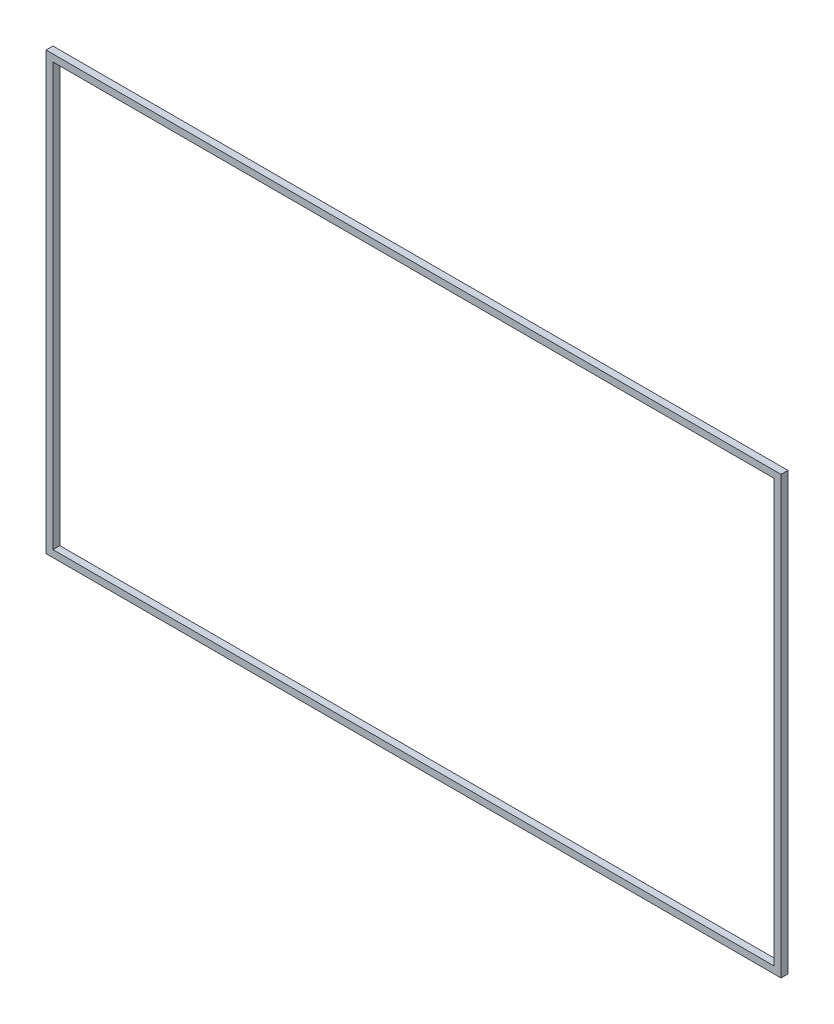
SolidWorks part; units mm, degrees
ref_plane "前视基准面" through (0, 0, 0) normal (0, 0, 1) x (1, 0, 0)
ref_plane "上视基准面" through (0, 0, 0) normal (0, 1, 0) x (1, 0, 0)
ref_plane "右视基准面" through (0, 0, 0) normal (1, 0, 0) x (0, 0, -1)
sketch "草图1" plane through (0, 0, 0) normal (0, 0, 1) x (1, 0, 0)
  line L0 (-477.3, -310.1) -> (477.3, -310.1) construction
  line L1 (-531, 5) -> (531, 5)
  line L3 (-521, -5) -> (521, -5)
  line L4 (531, 5) -> (531, -5)
  line L5 (-531, 5) -> (531, -5) construction
  line L8 (-531, 5) -> (-531, -625.2)
  line L11 (-477.3, -41.7) -> (-477.3, -578.5) construction
  line L13 (-531, -625.2) -> (531, -615.2) construction
  line L14 (-521, -5) -> (-521, -615.2)
  line L15 (531, -625.2) -> (531, -615.2)
  line L16 (-521, -615.2) -> (521, -615.2)
  line L18 (-531, -625.2) -> (531, -625.2)
  line L21 (-561, 24) -> (-561, -644) construction
  line L23 (0, 0) -> (0, -145.195) construction
  line L24 (531, -5) -> (531, -615.2)
  line L26 (521, -5) -> (521, -615.2)
  point P0 (0, 0)
  point P17 (-521, -615.2)
  point P18 (0, -620.2)
  dimension "D1" = 10
  dimension "D2" = 1062
  dimension "D3" = 10
  dimension "D4" = 30
  dimension "D5" = 10
  dimension "D6" = 10
  dimension "D7" = 10
extrude "凸台-拉伸1" add sketch "草图1" along normal blind 10
